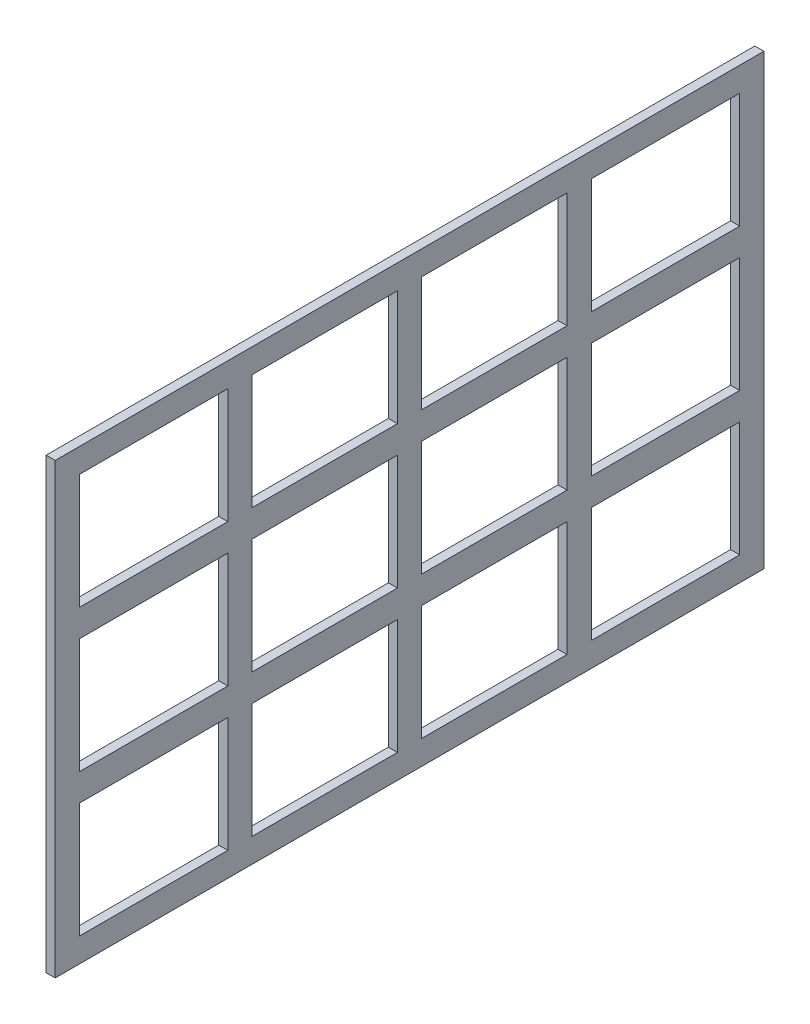
from build123d import *

# Parameters (mm, degrees)
SKETCH1_W           = 1170
SKETCH1_H           = 740
BOSS_EXTRUDE1_DEPTH = 7.5
SKETCH2_W           = 245
SKETCH2_H           = 190
SKETCH2_W_2         = 240
CUT_EXTRUDE1_DEPTH  = 108


with BuildPart() as part:
    # Sketch1 → Boss-Extrude1 (new, symmetric)
    with BuildSketch(Plane(origin=(0, 0, 0), x_dir=(0, 0, -1), z_dir=(1, 0, 0))):
        Rectangle(SKETCH1_W, SKETCH1_H)
    extrude(amount=BOSS_EXTRUDE1_DEPTH, both=True)

    # Sketch2 → Cut-Extrude1 (cut)
    with BuildSketch(Plane(origin=(7.5, 0, 0), x_dir=(0, 0, -1), z_dir=(1, 0, 0))):
        with Locations((-422.5, 235)):
            Rectangle(SKETCH2_W, SKETCH2_H)
        with Locations((-422.5, 0)):
            Rectangle(SKETCH2_W, SKETCH2_H)
        with Locations((-140, 0)):
            Rectangle(SKETCH2_W_2, SKETCH2_H)
        with Locations((-140, 235)):
            Rectangle(SKETCH2_W_2, SKETCH2_H)
        with Locations((-422.5, -235)):
            Rectangle(SKETCH2_W, SKETCH2_H)
        with Locations((-140, -235)):
            Rectangle(SKETCH2_W_2, SKETCH2_H)
    cut_extrude1 = extrude(amount=-CUT_EXTRUDE1_DEPTH, mode=Mode.SUBTRACT)

    # Mirror1: Cut-Extrude1 across plane
    add(cut_extrude1.mirror(Plane.XY), mode=Mode.SUBTRACT)


solid = part.part
